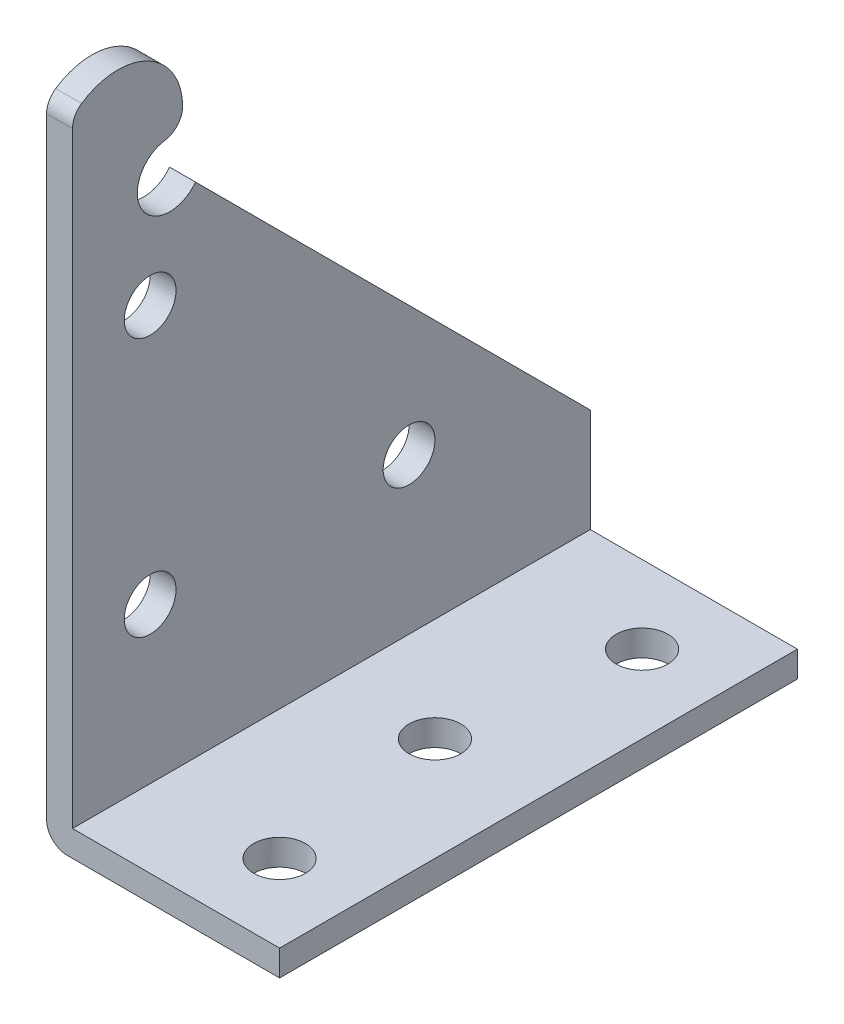
from build123d import *

# Parameters (mm, degrees)
SKETCH1_R           = 3.175
SKETCH1_W           = 63.5
SKETCH1_H           = 3.175
BOSS_EXTRUDE1_DEPTH = 3.175
SKETCH2_W           = 63.5
SKETCH2_H           = 3.175
BOSS_EXTRUDE2_DEPTH = 25.4
CUT_EXTRUDE1_DEPTH  = 106.992419611
SKETCH4_R           = 3.175
CUT_EXTRUDE2_DEPTH  = 25.4


with BuildPart() as part:
    # Sketch1 → Boss-Extrude1 (new body)
    # profile 1 of 2: a face of its own
    with BuildSketch(Plane(origin=(0, 0, 0), x_dir=(0, 0, -1), z_dir=(1, 0, 0))):
        with BuildLine():
            Line((0, 77.51210968), (0, 3.175))
            Line((0, 3.175), (63.5, 3.175))
            Line((63.5, 3.175), (63.5, 15.875))
            Line((63.5, 15.875), (15.080341671, 64.294658329))
            ThreePointArc((15.080341671, 64.294658329), (8.505408108, 64.65221549), (11.339511683, 70.595737627))
            ThreePointArc((11.339511683, 70.595737627), (12.906539417, 71.462906002), (13.511840983, 73.148482141))
            ThreePointArc((13.511840983, 73.148482141), (9.242521041, 80.072259125), (1.120938967, 79.618733943))
            ThreePointArc((1.120938967, 79.618733943), (0.297678098, 78.705253631), (0, 77.51210968))
        make_face()
        with Locations((9.525, 22.225)):
            Circle(SKETCH1_R, mode=Mode.SUBTRACT)
        with Locations((41.275, 22.225)):
            Circle(SKETCH1_R, mode=Mode.SUBTRACT)
        with Locations((9.525, 53.975)):
            Circle(SKETCH1_R, mode=Mode.SUBTRACT)
    # profile 2 of 2: a face of its own
    with BuildSketch(Plane(origin=(0, 0, 0), x_dir=(0, 0, -1), z_dir=(1, 0, 0))):
        with Locations((31.75, 1.5875)):
            Rectangle(SKETCH1_W, SKETCH1_H)
    extrude(amount=-BOSS_EXTRUDE1_DEPTH)

    # Sketch2 → Boss-Extrude2 (add)
    with BuildSketch(Plane(origin=(0, 0, 0), x_dir=(0, 0, -1), z_dir=(1, 0, 0))):
        with Locations((31.75, 1.5875)):
            Rectangle(SKETCH2_W, SKETCH2_H)
    extrude(amount=BOSS_EXTRUDE2_DEPTH)

    # Sketch3 → Cut-Extrude1 (cut, through all)
    with BuildSketch(Plane.XY):
        with BuildLine():
            ThreePointArc((-0.635, 0), (-2.431051224, 0.743948776), (-3.175, 2.54))
            Line((-3.175, 2.54), (-3.175, 0))
            Line((-3.175, 0), (-0.635, 0))
        make_face()
    extrude(amount=-CUT_EXTRUDE1_DEPTH, mode=Mode.SUBTRACT)

    # Sketch4 → Cut-Extrude2 (cut)
    with BuildSketch(Plane(origin=(0, 3.175, 0), x_dir=(1, 0, 0), z_dir=(0, 1, 0))):
        with Locations(Location((15.875, 53.975, 0), (0, 0, 270))):
            Circle(SKETCH4_R)
        with Locations(Location((12.7, 31.75, 0), (0, 0, 270))):
            Circle(SKETCH4_R)
        with Locations(Location((15.875, 9.525, 0), (0, 0, 270))):
            Circle(SKETCH4_R)
    extrude(amount=-CUT_EXTRUDE2_DEPTH, mode=Mode.SUBTRACT)


solid = part.part
